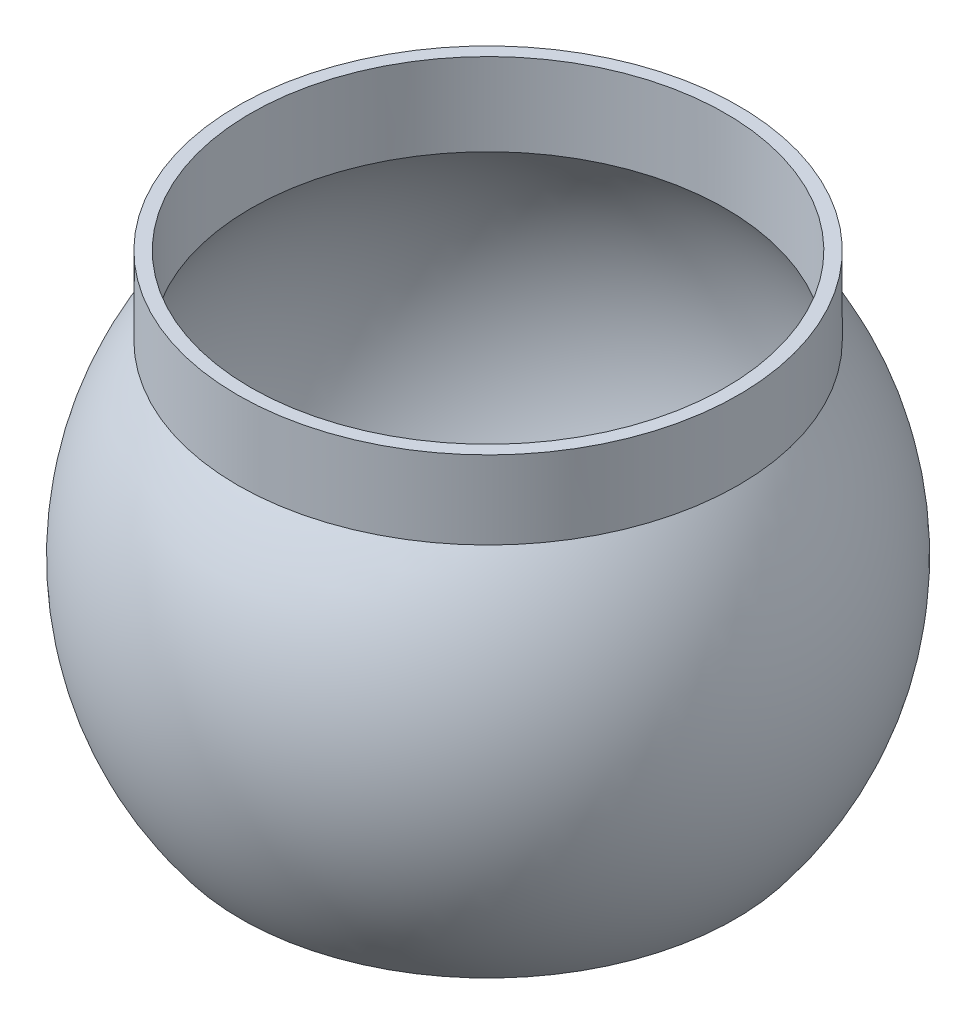
from build123d import *

# Parameters (mm, degrees)
SHELL_1_T = -2


with BuildPart() as part:
    # 草图1 → 旋转1 (revolve)
    with BuildSketch(Plane.XY, mode=Mode.PRIVATE) as revolve_1_sk:
        with BuildLine():
            Line((0, 0), (-38.5, 0))
            Line((-38.5, 0), (-38.5, -12))
            ThreePointArc((-38.5, -12), (-47.998171844, -41.085108941), (-37.993777534, -70))
            Line((-37.993777534, -70), (0, -70))
            Line((0, -70), (0, 0))
        make_face()
    revolve(revolve_1_sk.sketch.rotate(Axis((0, 0, 0), (0, -1, 0)), 270), axis=Axis((0, 0, 0), (0, -1, 0)))

    # 抽壳1
    shell_1_openings = [part.faces().sort_by_distance(p)[0] for p in [
        (0, -70, 0),
        (0, 0, 0),
    ]]
    offset(amount=SHELL_1_T, openings=shell_1_openings, kind=Kind.INTERSECTION)


solid = part.part
